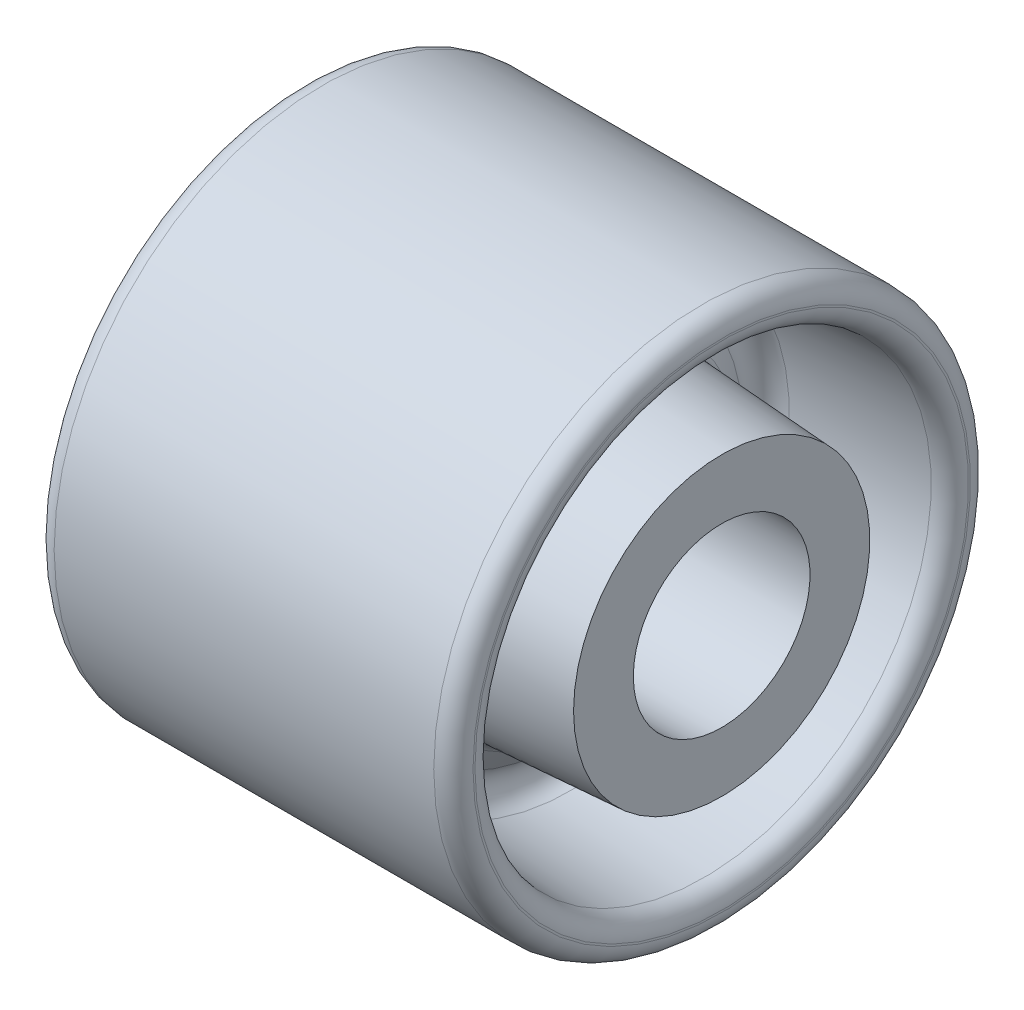
from build123d import *


with BuildPart() as part:
    # Sketch1 → Revolve1 (revolve)
    with BuildSketch(Plane(origin=(0, 0, 0), x_dir=(1, 0, 0), z_dir=(0, 1, 0)), mode=Mode.PRIVATE) as revolve1_sk:
        with BuildLine():
            Line((-35.418150087, 0), (28.581849913, 0))
            Line((28.581849913, 0), (28.581849913, 3))
            Line((28.581849913, 3), (28.581849913, 5.815314888))
            Line((28.581849913, 5.815314888), (28.581849913, 9.134334593))
            ThreePointArc((28.581849913, 9.134334593), (18.548299462, 9.927486707), (8.494011095, 10.388475153))
            ThreePointArc((8.494011095, 10.388475153), (7.284222242, 10.68234838), (6.297906579, 11.442040393))
            Line((6.297906579, 11.442040393), (3.297906579, 14.964563149))
            ThreePointArc((3.297906579, 14.964563149), (2.839777078, 18.126690149), (5.492050809, 19.90836741))
            ThreePointArc((5.492050809, 19.90836741), (15.695827227, 20.389287421), (25.877094288, 21.220033046))
            ThreePointArc((25.877094288, 21.220033046), (27.80510576, 22.191236773), (28.581849913, 24.20546949))
            Line((28.581849913, 24.20546949), (28.581849913, 24.5))
            ThreePointArc((28.581849913, 24.5), (27.703170256, 26.621320344), (25.581849913, 27.5))
            Line((25.581849913, 27.5), (-32.418150087, 27.5))
            ThreePointArc((-32.418150087, 27.5), (-34.539470431, 26.621320344), (-35.418150087, 24.5))
            Line((-35.418150087, 24.5), (-35.418150087, 24.20546949))
            ThreePointArc((-35.418150087, 24.20546949), (-34.641405934, 22.191236773), (-32.713394462, 21.220033046))
            ThreePointArc((-32.713394462, 21.220033046), (-22.532127402, 20.389287421), (-12.328350983, 19.90836741))
            ThreePointArc((-12.328350983, 19.90836741), (-11.119638388, 19.614127962), (-10.134206753, 18.854860232))
            Line((-10.134206753, 18.854860232), (-7.134206753, 15.332337476))
            ThreePointArc((-7.134206753, 15.332337476), (-6.676475178, 12.169314273), (-9.330311269, 10.388475153))
            ThreePointArc((-9.330311269, 10.388475153), (-22.394525119, 9.724589737), (-35.418150087, 8.5))
            Line((-35.418150087, 8.5), (-35.418150087, 5.815314888))
            Line((-35.418150087, 5.815314888), (-35.418150087, 3))
            Line((-35.418150087, 3), (-35.418150087, 0))
        make_face()
    revolve(revolve1_sk.sketch.rotate(Axis((-39.429457427, 0, 13.5), (1, 0, 0)), 180), axis=Axis((-39.429457427, 0, 13.5), (1, 0, 0)))


solid = part.part
